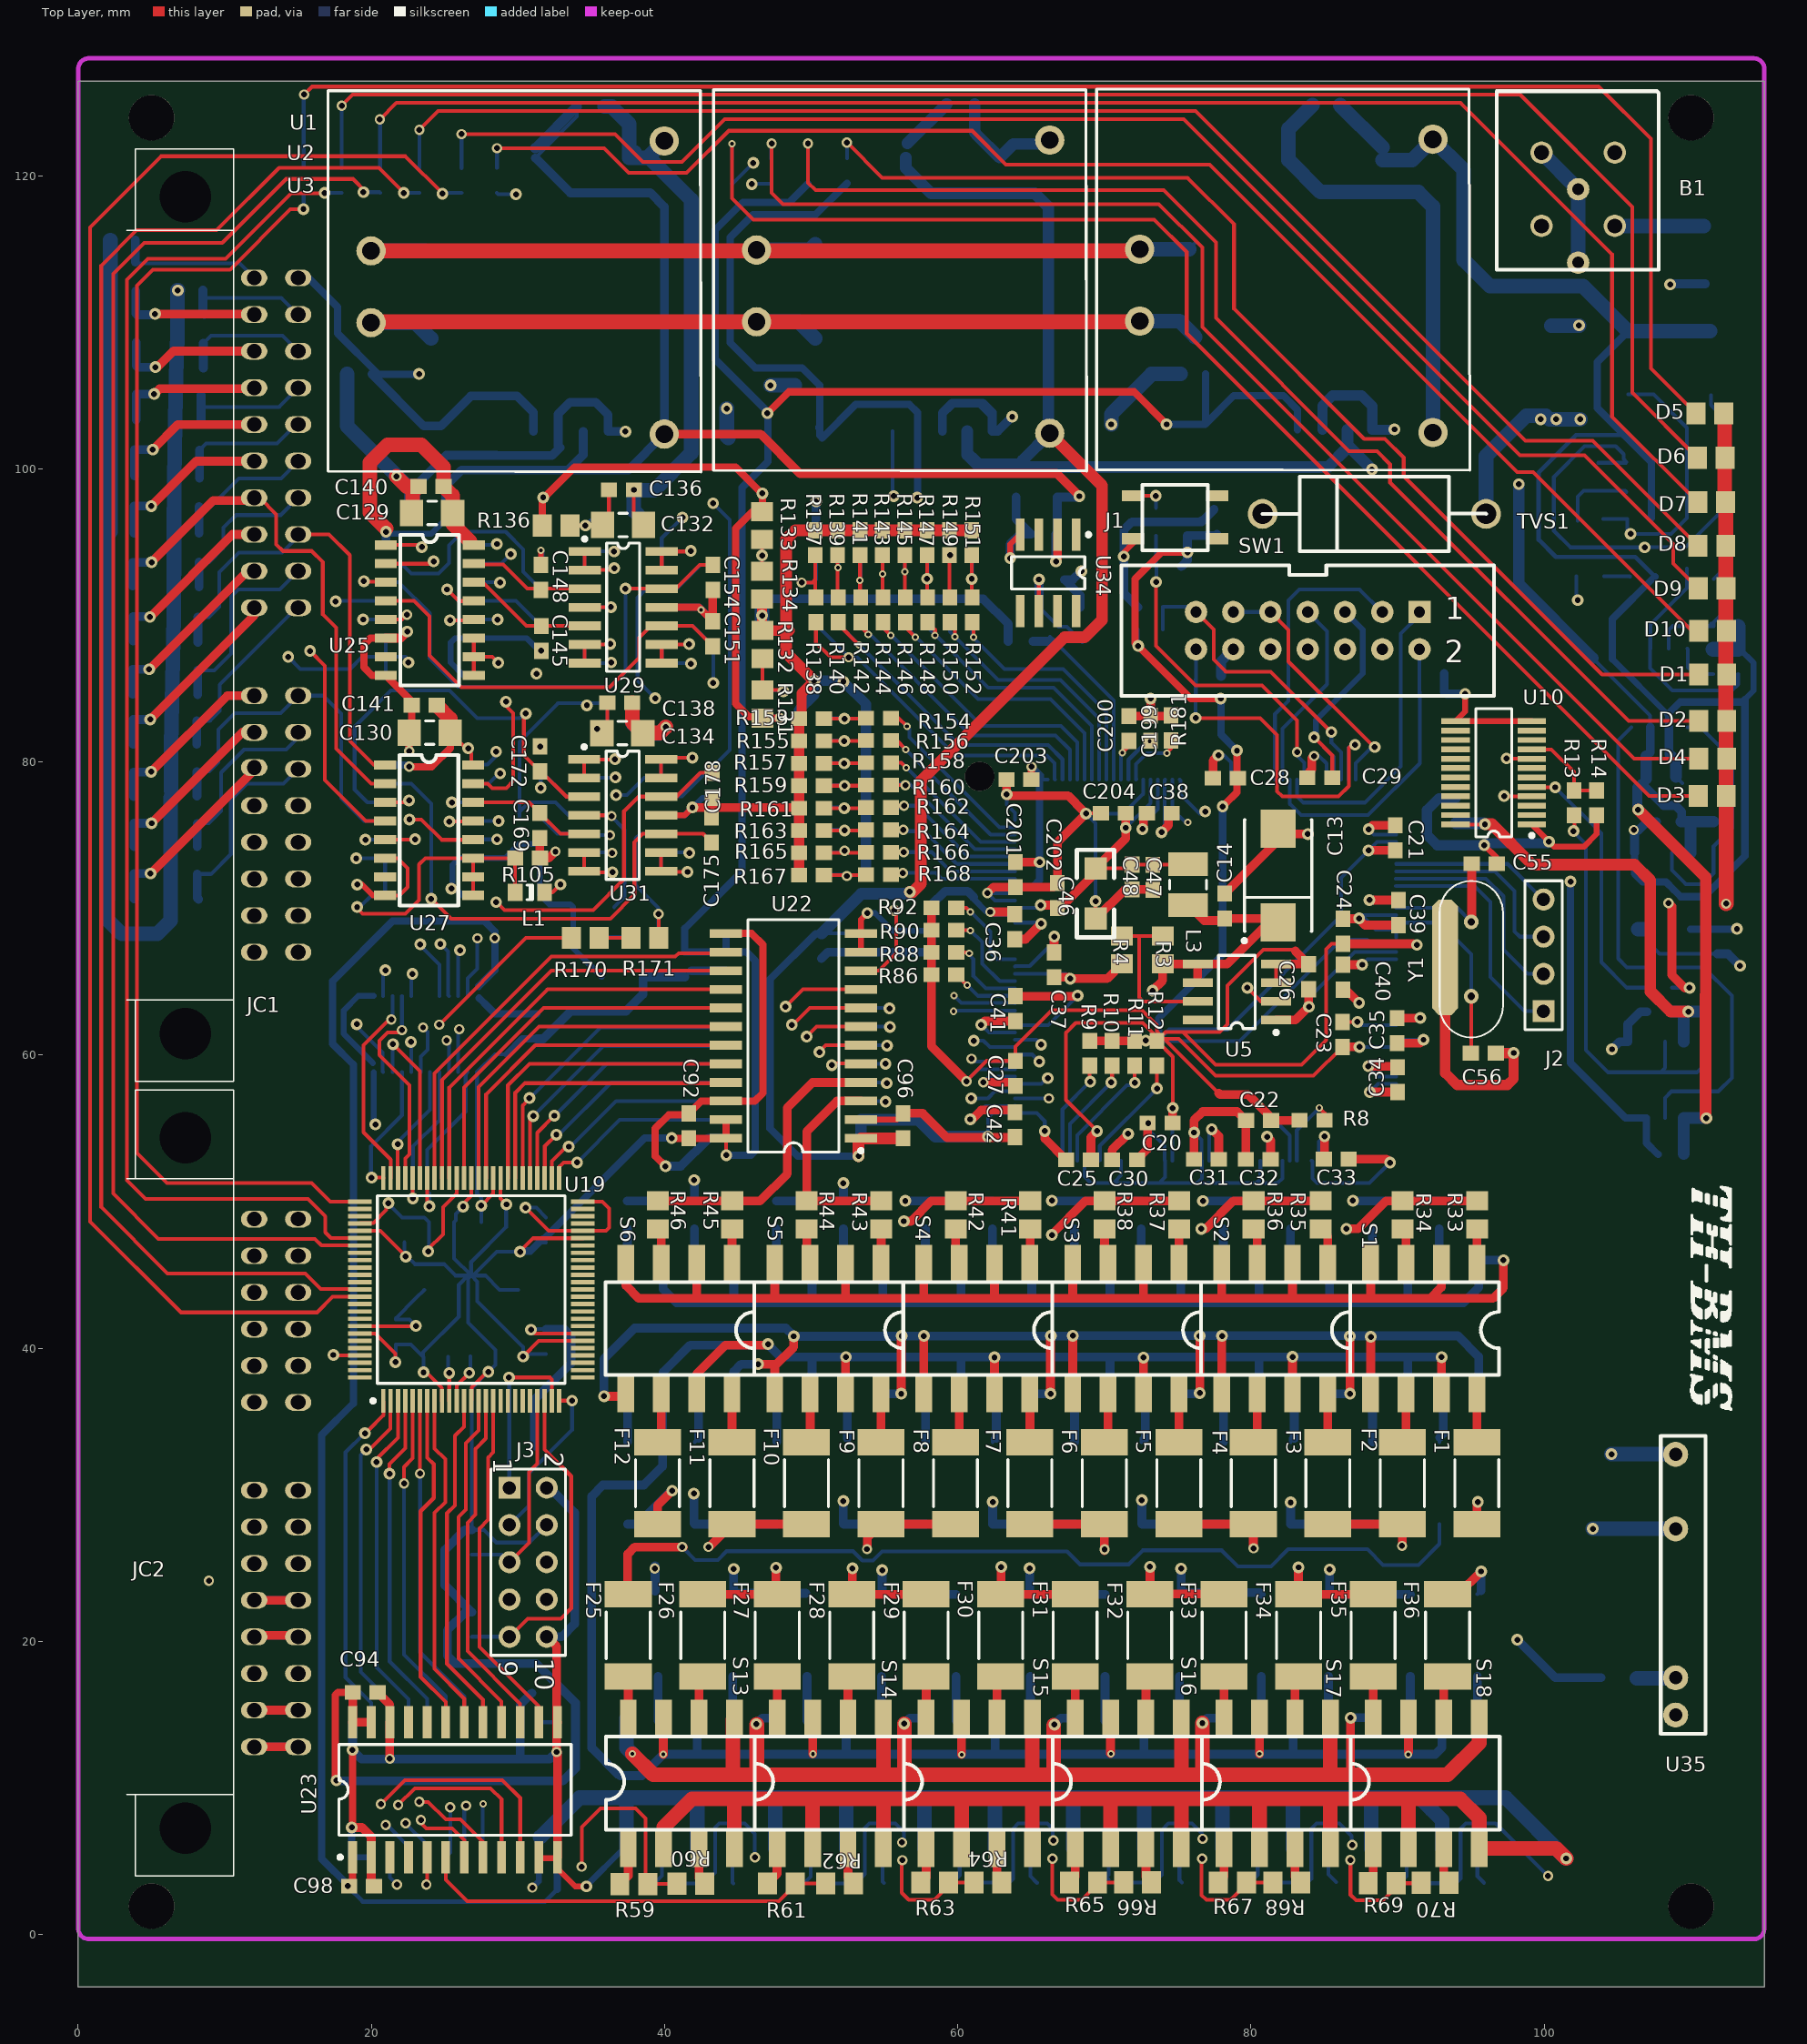
[diagram p0: Top Layer view]
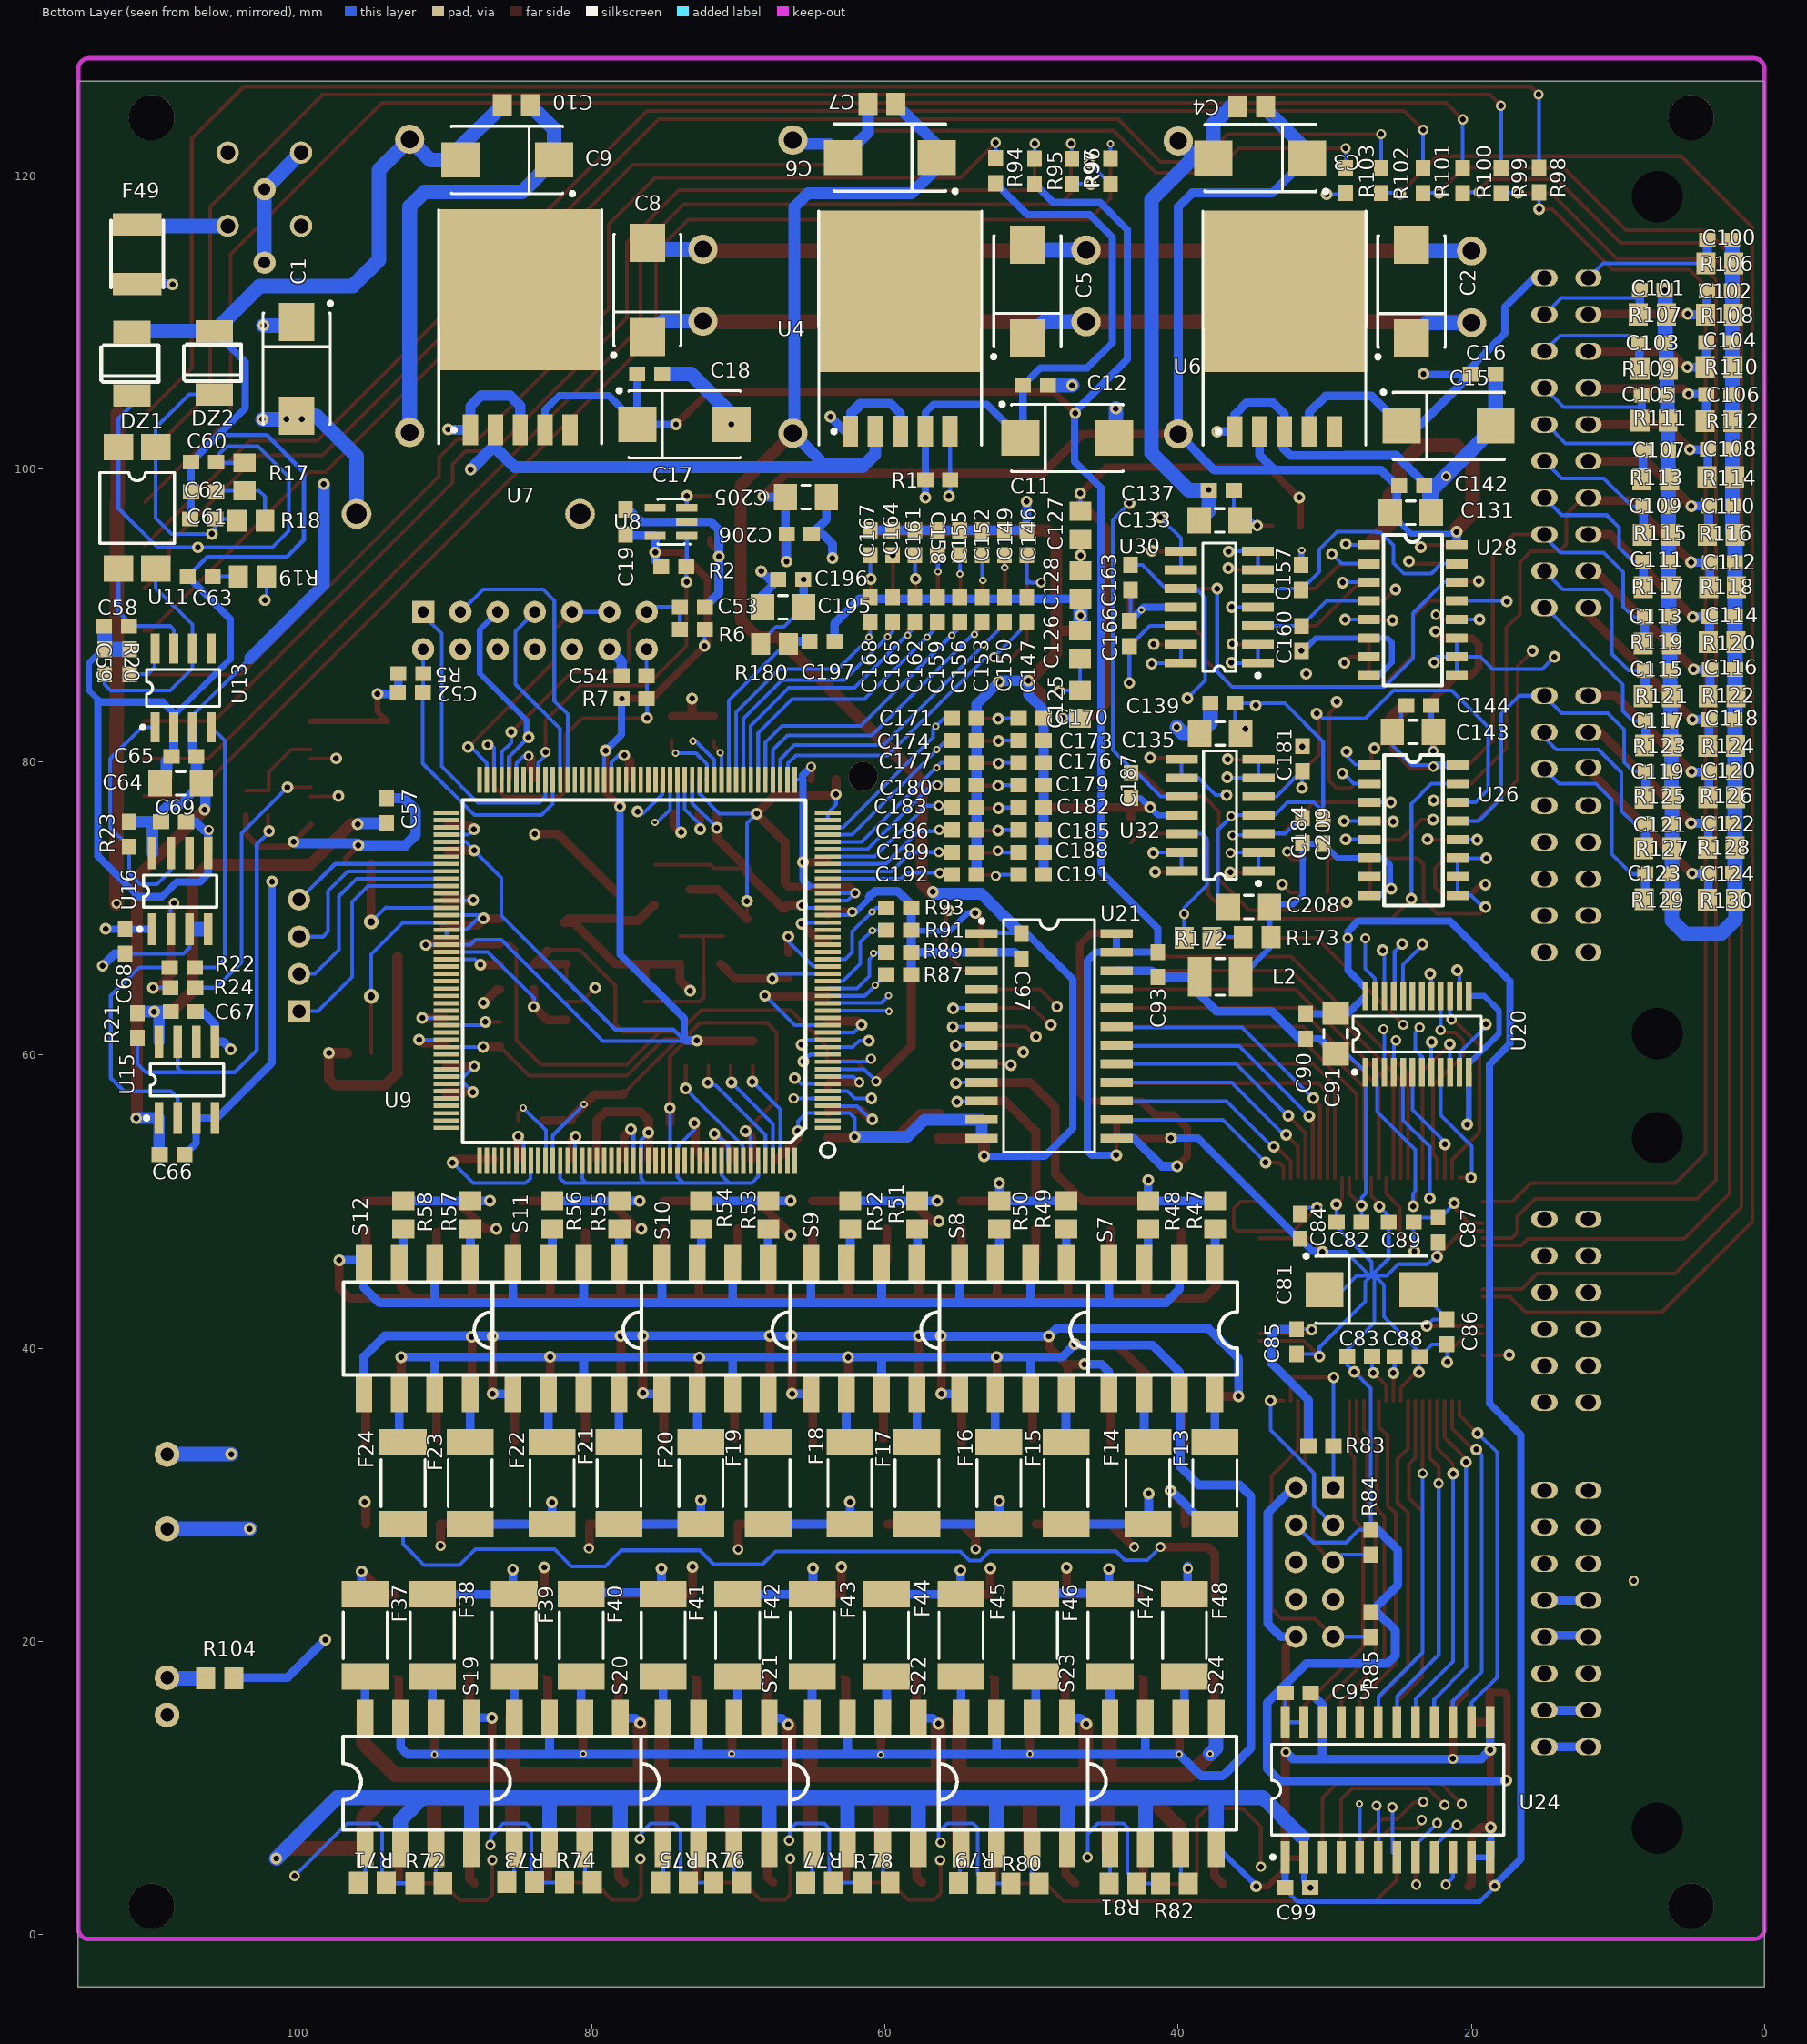
[diagram p1: Bottom Layer view, seen from below]
# Altium PCB MISC86180.PCBDOC (part 1 of 9)
Units mm, origin at the board's own origin, x right, y up, seen from the top; angles counter-clockwise.
Board outline 115 x 130 mm, 4 copper layers (Top Layer, GND, POWER, Bottom Layer); 475 components, 355 nets, 1755 pads, 459 vias.

## Layer stack, top to bottom (the 12.6 mil dielectric is the usual default, probably not edited)
Top Layer: signal copper 0.0356
Dielectric: core 0.32, FR-4, Dk 4.8
GND: signal copper 0.0356
Dielectric: prepreg 0.32, FR-4, Dk 4.8
POWER: signal copper 0.0356
Dielectric: core 0.32, FR-4, Dk 4.8
Bottom Layer: signal copper 0.0356

## Board outline
0.01,-3.55 115.01,-3.55 115.01,126.45 0.01,126.45

## Design rules (kind name [scope] priority, off if disabled: settings)
Clearance [All] p1: gap=0.3
PolygonConnect [All] p1: connectstyle=Relief reliefconductorwidth=0.254 reliefentries=4 polygonreliefangle="90 Angle"
RoutingVias [All] p1: holewidth=0.381 width=0.762 viastyle="Through Hole" minholewidth=0.305 minwidth=0.559 maxholewidth=5.08 maxwidth=6.858
SilkscreenOverComponentPads [All] p1: minsilkscreentomaskgap=0.254
SolderMaskExpansion [All] p1: expansion=0.102
TestPointUsage [All] p1: valid=0 allowmultiple=FALSE
Testpoint [All] p1: side=15 testpointundercomponent=TRUE minsize=1.016 maxsize=2.54 preferedsize=1.524 minholesize=0 maxholesize=1.016 preferedholesize=0.813 testpointgrid=0.025 style=1023 order=0-112345678
Width [All] p1: maxlimit=254 minlimit=0.254 preferedwidth=0.254
23 further rules are at their usual default settings.

## Components (designator, comment, footprint, x,y, rotation, side; value= is the part's Value field where it differs from the comment)
B1 "BNX012H" BNX012H 107.81,113.57 r270 top
C1 "Cap Pol3" TC7343-2917 100.1,106.83 r270 bottom
C2 "Cap Pol3" TC7343-2917 24.09,112.084 r90 bottom
C3 "Cap Pol3" TC7343-2917 34.38,121.19 r0 bottom
C4 "Cap" CR2012-0805 34.98,124.73 r180 bottom
C5 "Cap Pol3" TC7343-2917 50.29,112.094 r90 bottom
C6 "Cap Pol3" TC7343-2917 59.65,121.21 r0 bottom
C7 "Cap" CR2012-0805 60.21,124.91 r180 bottom
C8 "Cap Pol3" TC7343-2917 76.21,112.194 r90 bottom
C9 "Cap Pol3" TC7343-2917 85.75,121.05 r0 bottom
C10 "Cap" CR2012-0805 85.14,124.83 r180 bottom
C11 "Cap Pol3" TC7343-2917 47.56,102.12 r180 bottom
C12 "Cap" CR1608-0603 49.73,105.67 r0 bottom
C13 "Cap Pol3" TC7343-2917 81.83,72.25 r90 top
C14 "Cap" CR1608-0603 78.23,70.17 r270 top
C15 "Cap Pol3" TC7343-2917 21.55,102.94 r180 bottom
C16 "Cap" CR1608-0603 19.19,106.44 r0 bottom
C17 "Cap Pol3" TC7343-2917 73.67,103.05 r180 bottom
C18 "Cap" CR1608-0603 76.04,106.45 r0 bottom
C19 "Cap" CR1608-0603 77.654,96.376 r270 bottom
C20 "Cap" CR1608-0603 73.79,55.39 r0 top
C21 "Cap" CR1608-0603 89.85,74.83 r270 top
C22 "Cap" CR1608-0603 80.51,55.56 r0 top
C23 "Cap" CR1608-0603 86.25,61.41 r270 top
C24 "Cap" CR1608-0603 86.28,68.45 r270 top
C25 "Cap" CR1608-0603 68.23,52.88 r0 top
C26 "Cap" CR1608-0603 83.91,65.35 r90 top
C27 "Cap" CR1608-0603 63.91,58.76 r90 top
C28 "Cap" CR1608-0603 78.25,78.92 r0 top
C29 "Cap" CR1608-0603 84.69,78.94 r0 top
C30 "Cap" CR1608-0603 71.37,52.85 r180 top
C31 "Cap" CR1608-0603 76.95,52.92 r0 top
C32 "Cap" CR1608-0603 80.49,52.92 r0 top
C33 "Cap" CR1608-0603 85.81,52.89 r180 top
C34 "Cap" CR1608-0603 90,58.33 r270 top
C35 "Cap" CR1608-0603 89.95,61.67 r90 top
C36 "Cap" CR1608-0603 63.9,68.762 r270 top
C37 "Cap" CR1608-0603 66.55,66.16 r90 top
C38 "Cap" CR1608-0603 73.74,76.52 r0 top
C39 "Cap" CR1608-0603 90.04,69.72 r90 top
C40 "Cap" CR1608-0603 86.24,65.32 r90 top
C41 "Cap" CR1608-0603 63.9,63.174 r90 top
C42 "Cap" CR1608-0603 63.89,55.26 r90 top
C46 "Cap" 1206 69.39,69.3 r90 top
C47 "Cap" CR1608-0603 73.29,72.13 r90 top
C48 "Cap" CR1608-0603 71.87,72.15 r90 top
C52 "Cap" CR1608-0603 92.36,84.78 r180 bottom
C53 "Cap" CR1608-0603 73.122,90.538 r0 bottom
C54 "Cap" CR1608-0603 77.1,85.91 r180 bottom
C55 "Cap" CR1608-0603 95.9,73.043 r180 top
C56 "Cap" CR1608-0603 95.84,60.12 r180 top
C57 "Cap" CR1608-0603 93.95,76.68 r270 bottom
C58 "Cap" CR1608-0603 112.4,89.29 r180 bottom
C59 "Cap" CR1608-0603 113.2,86.84 r270 bottom
C60 "Cap" CR1608-0603 106.46,100.48 r180 bottom
C61 "Cap" CR1608-0603 106.52,96.6 r180 bottom
C62 "Cap" CR1608-0603 106.46,98.44 r180 bottom
C63 "Cap" CR1608-0603 106.69,92.668 r180 bottom
C64 "Cap" CR3216-1206 108.03,78.56 r180 bottom
C65 "Cap" CR1608-0603 107.8,80.4 r180 bottom
C66 "Cap" CR1608-0603 108.61,53.2 r0 bottom
C67 "Cap" CR1608-0603 107.85,62.95 r0 bottom
C68 "Cap" CR1608-0603 111.82,67.76 r90 bottom
C69 "Cap" CR1608-0603 108.51,75.91 r0 bottom
C81 "Cap Pol3" TC7343-2917 26.816,44.014 r180 bottom
C82 "Cap" CR1608-0603 28.34,48.586 r0 bottom
C83 "Cap" CR1608-0603 27.61,39.43 r0 bottom
C84 "Cap" CR1608-0603 31.66,48.32 r270 bottom
C85 "Cap" CR1608-0603 31.896,40.458 r270 bottom
C86 "Cap" CR1608-0603 21.64,41.12 r270 bottom
C87 "Cap" CR1608-0603 22.244,48.078 r270 bottom
C88 "Cap" CR1608-0603 24.38,39.44 r180 bottom
C89 "Cap" CR1608-0603 24.784,48.586 r0 bottom
C90 "Cap" CR1608-0603 31.306,61.966 r90 bottom
C91 "Cap" CR3216-1206 29.274,61.458 r90 bottom
C92 "Cap" CR1608-0603 41.68,55.18 r270 top
C93 "Cap" CR1608-0603 41.4,66.18 r90 bottom
C94 "Cap" CR1608-0603 19.58,16.51 r180 top
C95 "Cap" CR1608-0603 31.81,16.47 r0 bottom
C96 "Cap" CR1608-0603 56.29,55.18 r270 top
C97 "Cap" CR1608-0603 50.71,67.43 r90 bottom
C98 "Cap" CR1608-0603 19.33,3.29 r180 top
C99 "Cap" CR1608-0603 31.83,3.19 r0 bottom
C100 "Cap" CR1608-0603 3.05,115.58 r0 bottom
C101 "Cap" CR1608-0603 7.66,112.17 r0 bottom
C102 "Cap" CR1608-0603 3.079,112.118 r0 bottom
C103 "Cap" CR1608-0603 7.689,108.548 r0 bottom
C104 "Cap" CR1608-0603 3.12,108.6 r0 bottom
C105 "Cap" CR1608-0603 7.54,105 r0 bottom
C106 "Cap" CR1608-0603 3.12,105.07 r0 bottom
C107 "Cap" CR1608-0603 7.44,101.26 r0 bottom
C108 "Cap" CR1608-0603 3,101.3 r0 bottom
C109 "Cap" CR1608-0603 7.4,97.4 r0 bottom
C110 "Cap" CR1608-0603 2.96,97.44 r0 bottom
C111 "Cap" CR1608-0603 7.4,93.62 r0 bottom
C112 "Cap" CR1608-0603 2.87,93.59 r0 bottom
C113 "Cap" CR1608-0603 7.32,89.87 r0 bottom
C114 "Cap" CR1608-0603 2.89,89.9 r0 bottom
C115 "Cap" CR1608-0603 7.3,86.232 r0 bottom
C116 "Cap" CR1608-0603 2.86,86.298 r0 bottom
C117 "Cap" CR1608-0603 7.25,82.794 r0 bottom
C118 "Cap" CR1608-0603 2.92,82.88 r0 bottom
C119 "Cap" CR1608-0603 7.26,79.316 r0 bottom
C120 "Cap" CR1608-0603 2.94,79.292 r0 bottom
C121 "Cap" CR1608-0603 7.269,75.796 r0 bottom
C122 "Cap" CR1608-0603 2.97,75.804 r0 bottom
C123 "Cap" CR1608-0603 7.28,72.34 r0 bottom
C124 "Cap" CR1608-0603 2.98,72.38 r0 bottom
C125 "Cap" CR2012-0805 46.668,83.942 r270 bottom
C126 "Cap" CR2012-0805 46.668,88.006 r270 bottom
C127 "Cap" CR2012-0805 46.668,96.134 r90 bottom
C128 "Cap" CR2012-0805 46.668,92.07 r90 bottom
C129 "Cap" CR3216-1206 24.13,97.01 r0 top
C130 "Cap" CR3216-1206 23.972,82.024 r0 top
C131 "Cap" CR3216-1206 24.12,96.99 r0 bottom
C132 "Cap" CR3216-1206 37.174,96.144 r180 top
C133 "Cap" CR3216-1206 37.17,96.5 r180 bottom
C134 "Cap" CR3216-1206 37.134,81.958 r180 top
C135 "Cap" CR3216-1206 37.134,81.958 r180 bottom
C136 "Cap" CR1608-0603 37.054,98.546 r180 top
C137 "Cap" CR1608-0603 37.054,98.546 r180 bottom
C138 "Cap" CR1608-0603 36.944,84.03 r180 top
C139 "Cap" CR1608-0603 36.944,84.03 r180 bottom
C140 "Cap" CR1608-0603 24.07,98.816 r0 top
C141 "Cap" CR1608-0603 23.61,83.89 r0 top
C142 "Cap" CR1608-0603 24.07,98.816 r0 bottom
C143 "Cap" CR3216-1206 23.972,82.024 r0 bottom
C144 "Cap" CR1608-0603 23.59,83.85 r0 bottom
C145 "Cap" CR1608-0603 31.586,88.426 r90 top
C146 "Cap" CR1608-0603 50.302,94.954 r270 bottom
C147 "Cap" CR1608-0603 50.302,90.382 r270 bottom
C148 "Cap" CR1608-0603 31.586,92.588 r270 top
C149 "Cap" CR1608-0603 51.826,94.954 r270 bottom
C150 "Cap" CR1608-0603 51.826,90.382 r270 bottom
C151 "Cap" CR1608-0603 43.3,88.746 r270 top
C152 "Cap" CR1608-0603 53.35,94.954 r270 bottom
C153 "Cap" CR1608-0603 53.35,90.382 r270 bottom
C154 "Cap" CR1608-0603 43.27,92.588 r90 top
C155 "Cap" CR1608-0603 54.874,94.954 r270 bottom
C156 "Cap" CR1608-0603 54.874,90.382 r270 bottom
C157 "Cap" CR1608-0603 31.586,92.588 r270 bottom
C158 "Cap" CR1608-0603 56.398,94.954 r270 bottom
C159 "Cap" CR1608-0603 56.398,90.382 r270 bottom
C160 "Cap" CR1608-0603 31.586,88.426 r90 bottom
C161 "Cap" CR1608-0603 57.922,94.954 r270 bottom
C162 "Cap" CR1608-0603 57.922,90.382 r270 bottom
C163 "Cap" CR1608-0603 43.27,92.588 r90 bottom
C164 "Cap" CR1608-0603 59.446,94.954 r270 bottom
C165 "Cap" CR1608-0603 59.446,90.382 r270 bottom
C166 "Cap" CR1608-0603 43.3,88.746 r270 bottom
C167 "Cap" CR1608-0603 60.97,94.954 r270 bottom
C168 "Cap" CR1608-0603 60.97,90.382 r270 bottom
C169 "Cap" CR1608-0603 31.47,75.66 r90 top
C170 "Cap" CR1608-0603 50.018,82.97 r0 bottom
C171 "Cap" CR1608-0603 54.59,82.97 r0 bottom
C172 "Cap" CR1608-0603 31.53,80.21 r270 top
C173 "Cap" CR1608-0603 50.018,81.446 r0 bottom
C174 "Cap" CR1608-0603 54.59,81.446 r0 bottom
C175 "Cap" CR1608-0603 43.23,75.36 r270 top
C176 "Cap" CR1608-0603 50.018,79.922 r0 bottom
C177 "Cap" CR1608-0603 54.59,79.922 r0 bottom
C178 "Cap" CR1608-0603 43.23,78.402 r90 top
C179 "Cap" CR1608-0603 50.018,78.398 r0 bottom
C180 "Cap" CR1608-0603 54.59,78.398 r0 bottom
C181 "Cap" CR1608-0603 31.506,80.222 r270 bottom
C182 "Cap" CR1608-0603 50.018,76.874 r0 bottom
C183 "Cap" CR1608-0603 54.59,76.874 r0 bottom
C184 "Cap" CR1608-0603 31.52,75.32 r90 bottom
C185 "Cap" CR1608-0603 50.018,75.35 r0 bottom
C186 "Cap" CR1608-0603 54.59,75.35 r0 bottom
C187 "Cap" CR1608-0603 43.23,78.402 r90 bottom
C188 "Cap" CR1608-0603 50.018,73.826 r0 bottom
C189 "Cap" CR1608-0603 54.59,73.826 r0 bottom
C191 "Cap" CR1608-0603 50.018,72.302 r0 bottom
C192 "Cap" CR1608-0603 54.59,72.302 r0 bottom
C195 "Cap" CR3216-1206 66.95,90.57 r180 bottom
C196 "Cap" CR1608-0603 66.42,92.46 r180 bottom
C197 "Cap" CR1608-0603 64.28,88.21 r0 bottom
C199 "Cap" CR1608-0603 73.17,82.3 r270 top
C200 "Cap" CR1608-0603 71.69,82.28 r270 top
C201 "Cap" CR1608-0603 63.9,72.318 r90 top
C202 "Cap" CR1608-0603 66.81,70.89 r270 top
C203 "Cap" CR1608-0603 64.17,78.82 r0 top
C204 "Cap" CR1608-0603 70.61,76.51 r0 top
C205 "Cap" CR3216-1206 65.37,98.05 r0 bottom
C206 "Cap" CR1608-0603 65.84,95.53 r0 bottom
C208 "Cap" CR3216-1206 35.16,70.08 r0 bottom
C209 "Cap" CR1608-0603 30.12,75.27 r90 bottom
D1 "RED" CR2012-0805 111.48,85.98 r0 top
D2 "RED" CR2012-0805 111.48,82.81 r0 top
D3 "GREEN" CR2012-0805 111.45,77.7 r0 top
D4 "GREEN" CR2012-0805 111.48,80.24 r0 top
D5 "BLUE" CR2012-0805 111.29,103.79 r0 top
D6 "BLUE" CR2012-0805 111.38,100.77 r0 top
D7 "BLUE" CR2012-0805 111.4,97.75 r0 top
D8 "BLUE" CR2012-0805 111.42,94.76 r0 top
D9 "BLUE" CR2012-0805 111.44,91.86 r0 top
D10 "RED" CR2012-0805 111.46,88.97 r0 top
DZ1 "SMBJ8.5CA" AK_1B 111.36,109.33 r180 bottom
DZ2 "SMBJ8.5CA" AK_1B 105.72,109.39 r180 bottom
F1 "Res2" CR6332-2512 95.396,30.806 r90 top
F2 "Res2" CR6332-2512 90.316,30.806 r90 top
F3 "Res2" CR6332-2512 85.236,30.806 r90 top
F4 "Res2" CR6332-2512 80.156,30.806 r90 top
F5 "Res2" CR6332-2512 75.076,30.806 r90 top
F6 "Res2" CR6332-2512 69.996,30.806 r90 top
F7 "Res2" CR6332-2512 64.916,30.806 r90 top
F8 "Res2" CR6332-2512 59.836,30.806 r90 top
F9 "Res2" CR6332-2512 54.756,30.806 r90 top
F10 "Res2" CR6332-2512 49.676,30.806 r90 top
F11 "Res2" CR6332-2512 44.596,30.806 r90 top
F12 "Res2" CR6332-2512 39.516,30.806 r90 top
F13 "Res2" CR6332-2512 37.484,30.806 r90 bottom
F14 "Res2" CR6332-2512 42.056,30.806 r90 bottom
F15 "Res2" CR6332-2512 47.644,30.806 r90 bottom
F16 "Res2" CR6332-2512 52.216,30.806 r90 bottom
F17 "Res2" CR6332-2512 57.804,30.806 r90 bottom
F18 "Res2" CR6332-2512 62.376,30.806 r90 bottom
F19 "Res2" CR6332-2512 67.964,30.806 r90 bottom
F20 "Res2" CR6332-2512 72.536,30.806 r90 bottom
F21 "Res2" CR6332-2512 78.124,30.806 r90 bottom
F22 "Res2" CR6332-2512 82.696,30.806 r90 bottom
F23 "Res2" CR6332-2512 88.284,30.806 r90 bottom
F24 "Res2" CR6332-2512 92.856,30.806 r90 bottom
F25 "Res2" CR6332-2512 37.524,20.42 r270 top
F26 "Res2" CR6332-2512 42.604,20.42 r270 top
F27 "Res2" CR6332-2512 47.684,20.42 r270 top
F28 "Res2" CR6332-2512 52.764,20.42 r270 top
F29 "Res2" CR6332-2512 57.844,20.42 r270 top
F30 "Res2" CR6332-2512 62.924,20.42 r270 top
F31 "Res2" CR6332-2512 68.004,20.42 r270 top
F32 "Res2" CR6332-2512 73.084,20.42 r270 top
F33 "Res2" CR6332-2512 78.164,20.42 r270 top
F34 "Res2" CR6332-2512 83.244,20.42 r270 top
F35 "Res2" CR6332-2512 88.324,20.42 r270 top
F36 "Res2" CR6332-2512 93.404,20.42 r270 top
F37 "Res2" CR6332-2512 95.436,20.42 r270 bottom
F38 "Res2" CR6332-2512 90.864,20.42 r270 bottom
F39 "Res2" CR6332-2512 85.276,20.42 r270 bottom
F40 "Res2" CR6332-2512 80.704,20.42 r270 bottom
F41 "Res2" CR6332-2512 75.116,20.42 r270 bottom
F42 "Res2" CR6332-2512 70.036,20.42 r270 bottom
F43 "Res2" CR6332-2512 64.956,20.42 r270 bottom
F44 "Res2" CR6332-2512 59.876,20.42 r270 bottom
F45 "Res2" CR6332-2512 54.796,20.42 r270 bottom
F46 "Res2" CR6332-2512 49.716,20.42 r270 bottom
F47 "Res2" CR6332-2512 44.636,20.42 r270 bottom
F48 "Res2" CR6332-2512 39.556,20.42 r270 bottom
F49 "2.6A" FUSE 109.33,116.94 r270 bottom
J1 "JTAG_335" JTAG14 91.486,90.233 r180 top locked
J2 "Header 4" HDR1X4 99.95,63 r90 top
J3 "JTAG_CPLD" HDR2X5 29.42,30.49 r270 top